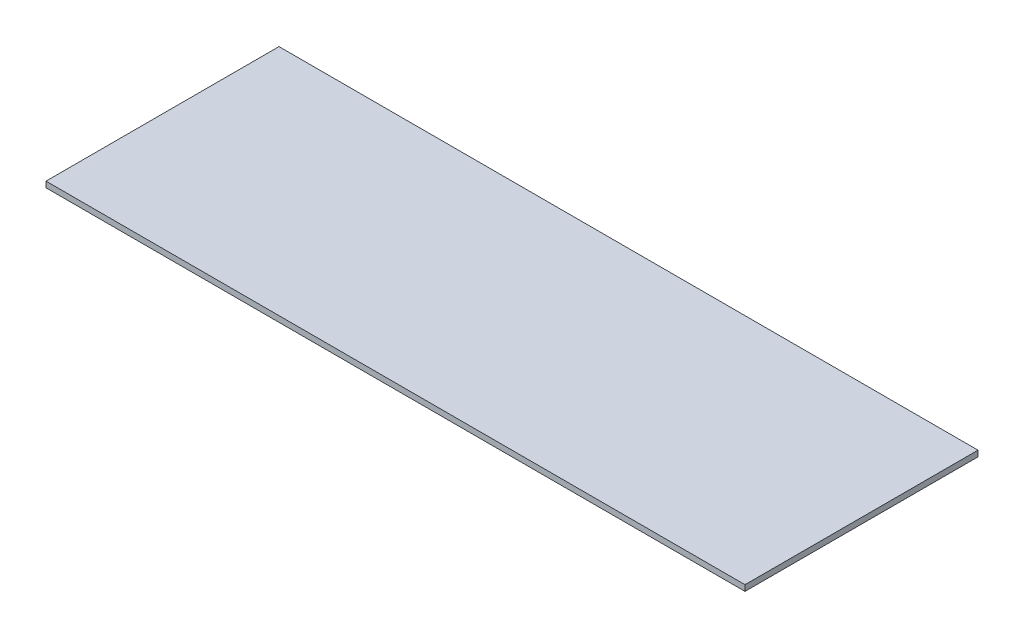
SolidWorks part; units mm, degrees
ref_plane "Front Plane" through (0, 0, 0) normal (0, 0, 1) x (1, 0, 0)
ref_plane "Top Plane" through (0, 0, 0) normal (0, 1, 0) x (1, 0, 0)
ref_plane "Right Plane" through (0, 0, 0) normal (1, 0, 0) x (0, 0, -1)
sketch "Sketch1" plane through (0, 0, 0) normal (0, 1, 0) x (1, 0, 0)
  line L1 (-600, 200) -> (600, 200)
  line L2 (-600, 200) -> (-600, -200)
  line L3 (-600, -200) -> (600, -200)
  line L4 (600, 200) -> (600, -200)
  line L5 (-600, 200) -> (600, -200) construction
  line L6 (-600, -200) -> (600, 200) construction
  point P0 (0, 0)
  dimension "D1" = 1200
  dimension "D2" = 400
extrude "Boss-Extrude1" add sketch "Sketch1" along normal blind 10
